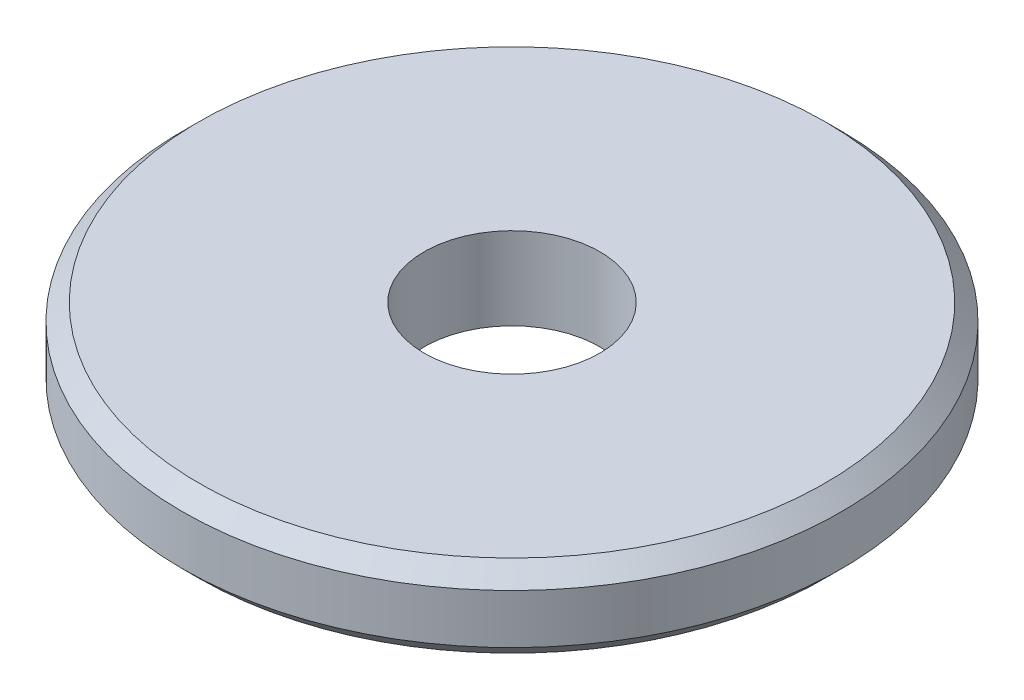
SolidWorks part; units mm, degrees
ref_plane "Front Plane" through (0, 0, 0) normal (0, 0, 1) x (1, 0, 0)
ref_plane "Top Plane" through (0, 0, 0) normal (0, 1, 0) x (1, 0, 0)
ref_plane "Right Plane" through (0, 0, 0) normal (1, 0, 0) x (0, 0, -1)
sketch "Sketch1" plane through (0, 0, 0) normal (0, 1, 0) x (1, 0, 0)
  circle A0 centre (0, 0) radius 1.6
  circle A1 centre (0, 0) radius 6
  dimension "D1" = 3.2
  dimension "D2" = 12
extrude "Boss-Extrude1" add sketch "Sketch1" along normal blind 1.5
chamfer "Chamfer1" distance 0.3 angle 45 2 edges at (0, 0, 6) (0, 1.5, 6)
